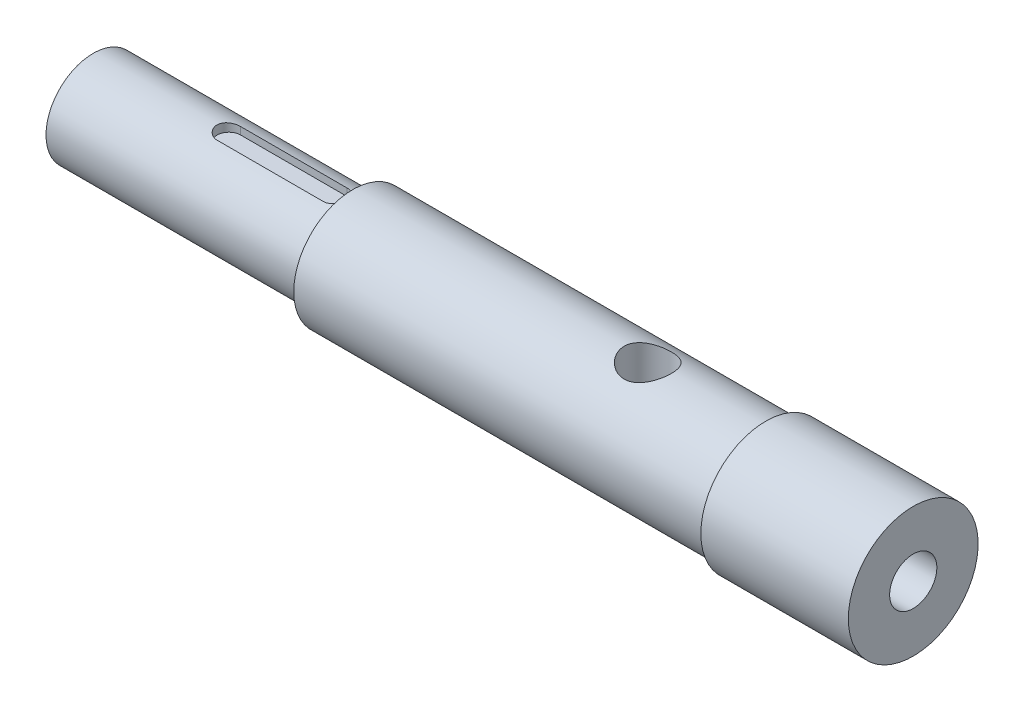
SolidWorks part; units mm, degrees
ref_plane "Front Plane" through (0, 0, 0) normal (0, 0, 1) x (1, 0, 0)
ref_plane "Top Plane" through (0, 0, 0) normal (0, 1, 0) x (1, 0, 0)
ref_plane "Right Plane" through (0, 0, 0) normal (1, 0, 0) x (0, 0, -1)
sketch "Sketch1" plane through (0, 0, 0) normal (0, 0, 1) x (1, 0, 0)
  line L0 (0, 0) -> (139, 0) construction
  line L1 (0, 8) -> (44, 8)
  line L2 (44, 8) -> (44, 10)
  line L3 (44, 10) -> (114, 10)
  line L4 (114, 10) -> (114, 11)
  line L5 (114, 11) -> (139, 11)
  line L6 (139, 11) -> (139, 4)
  line L7 (139, 4) -> (94, 4)
  line L8 (94, 4) -> (94, 0)
  line L9 (0, 8) -> (0, 0)
  line L10 (0, 0) -> (94, 0)
  dimension "D1" = 139
  dimension "D2" = 44
  dimension "D3" = 114
  dimension "D4" = 11
  dimension "D5" = 10
  dimension "D6" = 8
  dimension "D7" = 4
  dimension "D8" = 45
revolve "Revolve2" add sketch "Sketch1" angle 360 about L0
cosmetic thread "Cosmetic Thread1" parameters "D1"=45, "D2"=10
cosmetic thread "Cosmetic Thread2" parameters "D1"=20, "D2"=13.797
sketch "Sketch2" plane through (0, 0, 0) normal (0, 1, 0) x (1, 0, 0)
  line L0 (23, 0) -> (41, 0) construction
  line L1 (23, 2) -> (41, 2)
  line L2 (23, -2) -> (41, -2)
  line L3 (44, 8) -> (44, -8) construction
  arc A0 (23, 2) -> (23, -2) centre (23, 0) ccw
  arc A1 (41, -2) -> (41, 2) centre (41, 0) ccw
  point P3 (32, 0)
  point P8 (38.4283, 0)
  dimension "D1" = 2
  dimension "D2" = 18
  dimension "D3" = 3
extrude "Cut-Extrude1" cut sketch "Sketch2" against normal blind 1.5 from offset 8
sketch "Sketch3" plane through (0, 0, 0) normal (0, 1, 0) x (1, 0, 0)
  line L0 (139, -11) -> (139, 11) construction
  circle A0 centre (94, 0) radius 4
  dimension "D1" = 8
  dimension "D2" = 45
extrude "Cut-Extrude2" cut sketch "Sketch3" against normal through all both and the other way through all
